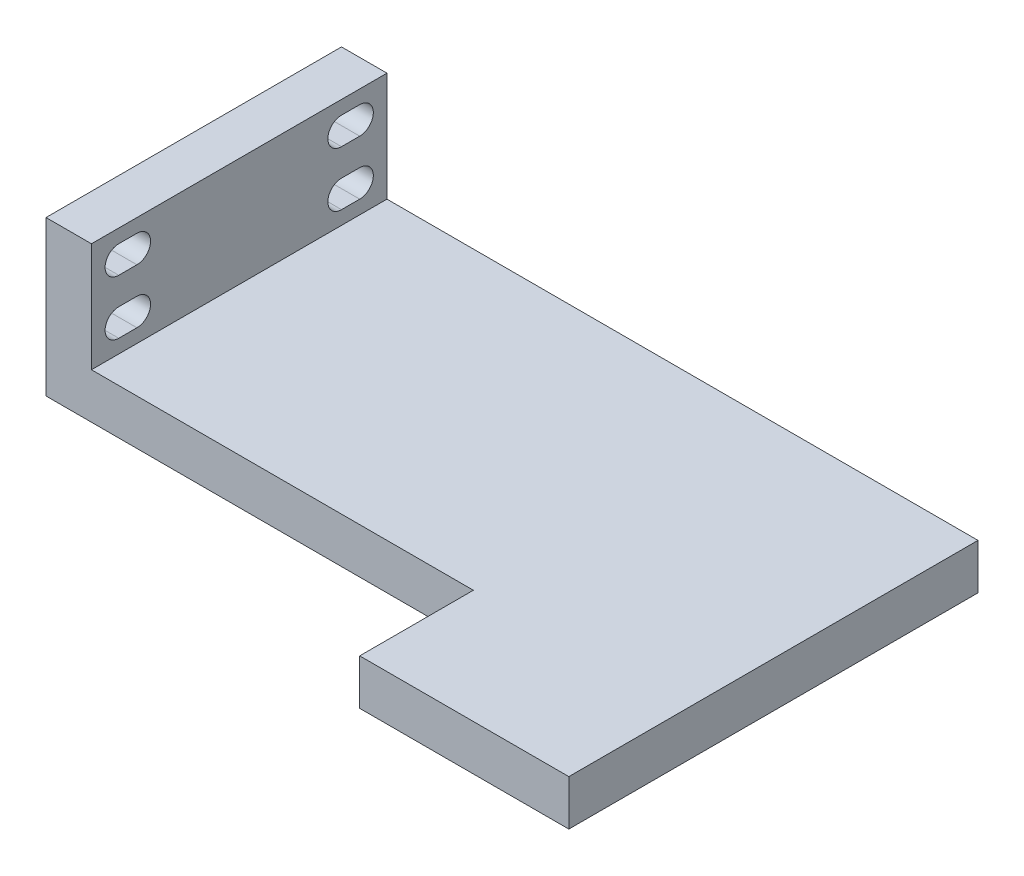
SolidWorks part; units mm, degrees
ref_plane "前视基准面" through (0, 0, 0) normal (0, 0, 1) x (1, 0, 0)
ref_plane "上视基准面" through (0, 0, 0) normal (0, 1, 0) x (1, 0, 0)
ref_plane "右视基准面" through (0, 0, 0) normal (1, 0, 0) x (0, 0, -1)
sketch "草图1" plane through (0, 0, 0) normal (0, 0, 1) x (1, 0, 0)
  line L0 (0, 0) -> (0, 34)
  line L1 (0, 34) -> (10, 34)
  line L2 (10, 34) -> (10, 10)
  line L3 (10, 10) -> (140, 10)
  line L4 (140, 10) -> (140, 0)
  line L5 (140, 0) -> (0, 0)
  dimension "D1" = 10
  dimension "D2" = 24
  dimension "D3" = 10
  dimension "D4" = 130
extrude "凸台-拉伸1" add sketch "草图1" along normal mid plane 65
sketch "草图2" plane through (10, 0, 0) normal (1, 0, 0) x (0, 0, -1)
  line L0 (-26.5, 28) -> (-22.5, 28) construction
  line L1 (-26.5, 31) -> (-22.5, 31)
  line L2 (-26.5, 25) -> (-22.5, 25)
  line L3 (22.5, 28) -> (26.5, 28) construction
  line L4 (22.5, 31) -> (26.5, 31)
  line L5 (22.5, 25) -> (26.5, 25)
  line L6 (-32.5, 10) -> (-32.5, 34) construction
  line L7 (32.5, 10) -> (32.5, 34) construction
  line L8 (-32.5, 34) -> (32.5, 34) construction
  line L9 (32.5, 22) -> (-32.5, 22) construction
  line L10 (-26.5, 16) -> (-22.5, 16) construction
  line L11 (-26.5, 13) -> (-22.5, 13)
  line L12 (-26.5, 19) -> (-22.5, 19)
  line L13 (22.5, 16) -> (26.5, 16) construction
  line L14 (22.5, 13) -> (26.5, 13)
  line L15 (22.5, 19) -> (26.5, 19)
  arc A0 (-26.5, 31) -> (-26.5, 25) centre (-26.5, 28) ccw
  arc A1 (-22.5, 25) -> (-22.5, 31) centre (-22.5, 28) ccw
  arc A2 (22.5, 31) -> (22.5, 25) centre (22.5, 28) ccw
  arc A3 (26.5, 25) -> (26.5, 31) centre (26.5, 28) ccw
  arc A4 (-26.5, 13) -> (-26.5, 19) centre (-26.5, 16) cw
  arc A5 (-22.5, 19) -> (-22.5, 13) centre (-22.5, 16) cw
  arc A6 (22.5, 13) -> (22.5, 19) centre (22.5, 16) cw
  arc A7 (26.5, 19) -> (26.5, 13) centre (26.5, 16) cw
  point P2 (-24.5, 28)
  point P8 (24.5, 28)
  point P24 (-24.5, 16)
  point P31 (24.5, 16)
extrude "切除-拉伸1" cut sketch "草图2" against normal up to next
sketch "草图3" plane through (0, 10, 0) normal (0, 1, 0) x (1, 0, 0)
  line L0 (140, -32.5) -> (140, 32.5) construction
  line L1 (140, -57.5) -> (94, -57.5)
  line L2 (140, -57.5) -> (140, -32.5)
  line L3 (140, -32.5) -> (94, -32.5)
  line L4 (94, -57.5) -> (94, -32.5)
  line L5 (140, -32.5) -> (10, -32.5) construction
  point P5 (0, 0)
  point P6 (0, 0)
  point P7 (140, -32.5)
  point P10 (94, -32.5)
  dimension "D1" = 46
  dimension "D2" = 25
extrude "凸台-拉伸2" add sketch "草图3" against normal up to surface (10 mm away) up to face at (70, 0, 0)
equation "\"D3@草图2\"=\"D2@草图2\""
